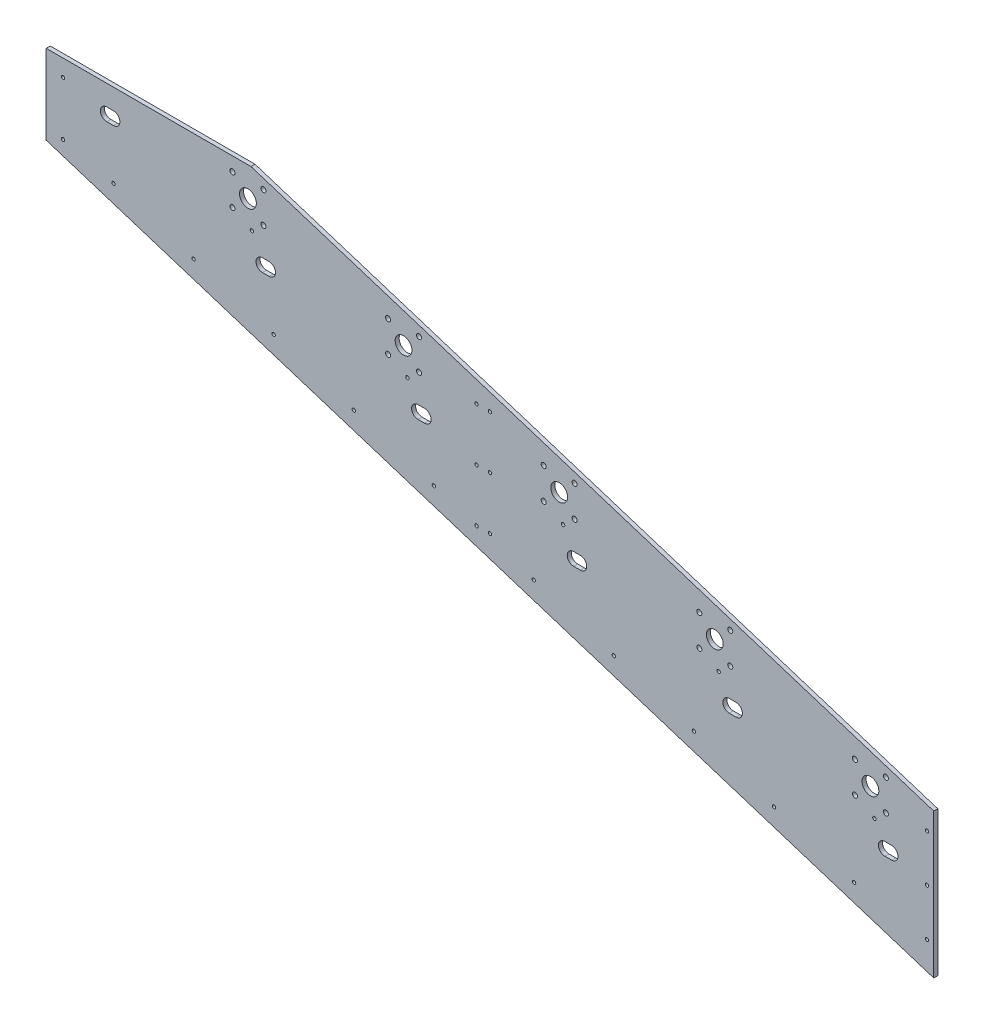
from build123d import *

# Parameters (mm, degrees)
SKETCH_1_W             = 3700
SKETCH_1_H             = 1176
EXTRUDE_1_DEPTH        = 12
SKETCH_2_R             = 19
SKETCH_2_R_2           = 25
CUT_EXTRUDE_1_DEPTH    = 4036.525368524
PATTERN_LINEAR_1_COUNT = 5
PATTERN_LINEAR_1_PITCH = 485.711841895
CUT_EXTRUDE_2_DEPTH    = 4036.525368524
CUT_EXTRUDE_4_DEPTH    = 4036.525368524
CUT_EXTRUDE_5_DEPTH    = 4036.525368524
PATTERN_LINEAR_2_COUNT = 6
PATTERN_LINEAR_2_PITCH = 485.711841895
SKETCH_9_R             = 7.5
CUT_EXTRUDE_11_DEPTH   = 4036.525368524
SKETCH_11_R            = 5
CUT_EXTRUDE_12_DEPTH   = 4036.525368524
PATTERN_LINEAR_3_COUNT = 5
PATTERN_LINEAR_3_PITCH = 485.711841895
SKETCH_12_R            = 5
CUT_EXTRUDE_13_DEPTH   = 3093.743927324
PATTERN_LINEAR_4_COUNT = 5
PATTERN_LINEAR_4_PITCH = 485.711841895
EXTRUDE_4_DEPTH        = 12
CUT_EXTRUDE_14_DEPTH   = 3093.743927324
PATTERN_LINEAR_5_COUNT = 4
PATTERN_LINEAR_5_PITCH = 485.711841895


with BuildPart() as part:
    # 草图1 → 凸台-拉伸1 (new body)
    with BuildSketch(Plane.XY.offset(-510)):
        with Locations((1850, 1023)):
            Rectangle(SKETCH_1_W, SKETCH_1_H)
    extrude(amount=EXTRUDE_1_DEPTH)

    # 草图2 → 切除-拉伸1 (cut, through all)
    with BuildSketch(Plane(origin=(0, 0, -510), x_dir=(-1, 0, 0), z_dir=(0, 0, -1))):
        with Locations((-200, 1531)):
            Circle(SKETCH_2_R)
        with Locations((-599.939078063, 1524.019037425)):
            Circle(SKETCH_2_R_2)
    cut_extrude_1 = extrude(amount=-CUT_EXTRUDE_1_DEPTH, mode=Mode.SUBTRACT)

    # 阵列(线性)1: 切除-拉伸1 ×5
    with Locations(*[Vector(0.9531146620938385, -0.30260938667157716, 0) * (i * PATTERN_LINEAR_1_PITCH) for i in range(1, PATTERN_LINEAR_1_COUNT)]):
        add(cut_extrude_1, mode=Mode.SUBTRACT)

    # 草图5 → 切除-拉伸2 (cut, through all)
    with BuildSketch(Plane(origin=(0, 0, -510), x_dir=(-1, 0, 0), z_dir=(0, 0, -1))):
        Polygon((-608.945764682, 1611), (-3700, 629.604934412), (-3700, 1611), align=None)
    extrude(amount=-CUT_EXTRUDE_2_DEPTH, mode=Mode.SUBTRACT)

    # 草图6 → 切除-拉伸4 (cut, through all)
    with BuildSketch(Plane(origin=(0, 0, -510), x_dir=(-1, 0, 0), z_dir=(0, 0, -1))):
        Polygon((-2958.056115955, 435), (0, 1374.16879321), (0, 435), align=None)
    extrude(amount=-CUT_EXTRUDE_4_DEPTH, mode=Mode.SUBTRACT)

    # 草图7 → 切除-拉伸5 (cut, through all)
    with BuildSketch(Plane(origin=(0, 0, -510), x_dir=(-1, 0, 0), z_dir=(0, 0, -1))):
        with BuildLine():
            Line((-200, 1550), (-180, 1550))
            ThreePointArc((-180, 1550), (-161, 1531), (-180, 1512))
            Line((-180, 1512), (-200, 1512))
            ThreePointArc((-200, 1512), (-219, 1531), (-200, 1550))
        make_face()
    cut_extrude_5 = extrude(amount=-CUT_EXTRUDE_5_DEPTH, mode=Mode.SUBTRACT)

    # 阵列(线性)2: 切除-拉伸5 ×6
    with Locations(*[Vector(0.9531146620938385, -0.30260938667157716, 0) * (i * PATTERN_LINEAR_2_PITCH) for i in range(1, PATTERN_LINEAR_2_COUNT)]):
        add(cut_extrude_5, mode=Mode.SUBTRACT)

    # 草图9 → 切除-拉伸11 (cut, through all)
    with BuildSketch(Plane(origin=(0, 0, -510), x_dir=(-1, 0, 0), z_dir=(0, 0, -1))):
        with Locations((-553.939078063, 1570.019037425)):
            Circle(SKETCH_9_R)
        with Locations((-645.939078063, 1570.019037425)):
            Circle(SKETCH_9_R)
        with Locations((-645.939078063, 1478.019037425)):
            Circle(SKETCH_9_R)
        with Locations((-553.939078063, 1478.019037425)):
            Circle(SKETCH_9_R)
    cut_extrude_11 = extrude(amount=-CUT_EXTRUDE_11_DEPTH, mode=Mode.SUBTRACT)

    # 草图11 → 切除-拉伸12 (cut, through all)
    with BuildSketch(Plane(origin=(0, 0, -510), x_dir=(-1, 0, 0), z_dir=(0, 0, -1))):
        with Locations((-2403.114662094, 663.650866112)):
            Circle(SKETCH_11_R)
        with Locations((-50, 1561)):
            Circle(SKETCH_11_R)
        with Locations((-50, 1401)):
            Circle(SKETCH_11_R)
        with Locations((-200, 1363.129326761)):
            Circle(SKETCH_11_R)
        with Locations((-438.278665523, 1287.476980093)):
            Circle(SKETCH_11_R)
        with Locations((-676.557331047, 1211.824633425)):
            Circle(SKETCH_11_R)
        with Locations((-914.83599657, 1136.172286757)):
            Circle(SKETCH_11_R)
        with Locations((-1153.114662094, 1060.519940089)):
            Circle(SKETCH_11_R)
        with Locations((-1280, 1021)):
            Circle(SKETCH_11_R)
        with Locations((-1320, 1021)):
            Circle(SKETCH_11_R)
        with Locations((-1280, 1178)):
            Circle(SKETCH_11_R)
        with Locations((-1320, 1178)):
            Circle(SKETCH_11_R)
        with Locations((-1320, 1335)):
            Circle(SKETCH_11_R)
        with Locations((-1280, 1335)):
            Circle(SKETCH_11_R)
        with Locations((-1450, 966.260252783)):
            Circle(SKETCH_11_R)
        with Locations((-1688.278665523, 890.607906115)):
            Circle(SKETCH_11_R)
        with Locations((-1926.557331047, 814.955559447)):
            Circle(SKETCH_11_R)
        with Locations((-2164.83599657, 739.30321278)):
            Circle(SKETCH_11_R)
        with Locations((-2620, 625)):
            Circle(SKETCH_11_R)
        with Locations((-2620, 765)):
            Circle(SKETCH_11_R)
        with Locations((-2620, 905)):
            Circle(SKETCH_11_R)
    extrude(amount=-CUT_EXTRUDE_12_DEPTH, mode=Mode.SUBTRACT)

    # 阵列(线性)3: 切除-拉伸11 ×5
    with Locations(*[Vector(0.9531146620938385, -0.30260938667157716, 0) * (i * PATTERN_LINEAR_3_PITCH) for i in range(1, PATTERN_LINEAR_3_COUNT)]):
        add(cut_extrude_11, mode=Mode.SUBTRACT)

    # Surface Cut 1
    split(bisect_by=Plane.ZY.offset(-2640), keep=Keep.TOP)

    # 草图12 → 切除-拉伸13 (cut, through all)
    with BuildSketch(Plane(origin=(0, 0, -510), x_dir=(-1, 0, 0), z_dir=(0, 0, -1))):
        with Locations((-611.679078063, 1446.789037425)):
            Circle(SKETCH_12_R)
    cut_extrude_13 = extrude(amount=-CUT_EXTRUDE_13_DEPTH, mode=Mode.SUBTRACT)

    # 阵列(线性)4: 切除-拉伸13 ×5
    with Locations(*[Vector(0.9531146620938385, -0.3026093866715771, 0) * (i * PATTERN_LINEAR_4_PITCH) for i in range(1, PATTERN_LINEAR_4_COUNT)]):
        add(cut_extrude_13, mode=Mode.SUBTRACT)

    # 草图15 → 凸台-拉伸4 (add, through all)
    with BuildSketch(Plane(origin=(0, 0, -510), x_dir=(-1, 0, 0), z_dir=(0, 0, -1))):
        with BuildLine():
            Line((-662.939078063, 1414.019037425), (-642.939078063, 1414.019037425))
            ThreePointArc((-642.939078063, 1414.019037425), (-612.939078063, 1384.019037425), (-642.939078063, 1354.019037425))
            Line((-642.939078063, 1354.019037425), (-662.939078063, 1354.019037425))
            ThreePointArc((-662.939078063, 1354.019037425), (-692.939078063, 1384.019037425), (-662.939078063, 1414.019037425))
        make_face()
        with BuildLine():
            Line((-1125.878156125, 1267.03807485), (-1105.878156125, 1267.03807485))
            ThreePointArc((-1105.878156125, 1267.03807485), (-1075.878156125, 1237.03807485), (-1105.878156125, 1207.03807485))
            Line((-1105.878156125, 1207.03807485), (-1125.878156125, 1207.03807485))
            ThreePointArc((-1125.878156125, 1207.03807485), (-1155.878156125, 1237.03807485), (-1125.878156125, 1267.03807485))
        make_face()
        with BuildLine():
            Line((-1588.817234188, 1120.057112275), (-1568.817234188, 1120.057112275))
            ThreePointArc((-1568.817234188, 1120.057112275), (-1538.817234188, 1090.057112275), (-1568.817234188, 1060.057112275))
            Line((-1568.817234188, 1060.057112275), (-1588.817234188, 1060.057112275))
            ThreePointArc((-1588.817234188, 1060.057112275), (-1618.817234188, 1090.057112275), (-1588.817234188, 1120.057112275))
        make_face()
        with BuildLine():
            Line((-2051.75631225, 973.0761497), (-2031.75631225, 973.0761497))
            ThreePointArc((-2031.75631225, 973.0761497), (-2001.75631225, 943.0761497), (-2031.75631225, 913.0761497))
            Line((-2031.75631225, 913.0761497), (-2051.75631225, 913.0761497))
            ThreePointArc((-2051.75631225, 913.0761497), (-2081.75631225, 943.0761497), (-2051.75631225, 973.0761497))
        make_face()
    extrude(amount=-EXTRUDE_4_DEPTH)

    # 草图14 → 切除-拉伸14 (cut, through all)
    with BuildSketch(Plane(origin=(0, 0, -510), x_dir=(-1, 0, 0), z_dir=(0, 0, -1))):
        with BuildLine():
            Line((-642.939078063, 1393.019037425), (-662.939078063, 1393.019037425))
            ThreePointArc((-662.939078063, 1393.019037425), (-681.939078063, 1374.019037425), (-662.939078063, 1355.019037425))
            Line((-662.939078063, 1355.019037425), (-642.939078063, 1355.019037425))
            ThreePointArc((-642.939078063, 1355.019037425), (-623.939078063, 1374.019037425), (-642.939078063, 1393.019037425))
        make_face()
    cut_extrude_14 = extrude(amount=-CUT_EXTRUDE_14_DEPTH, mode=Mode.SUBTRACT)

    # 阵列(线性)5: 切除-拉伸14 ×4
    with Locations(*[Vector(0.9531146620938385, -0.3026093866715771, 0) * (i * PATTERN_LINEAR_5_PITCH) for i in range(1, PATTERN_LINEAR_5_COUNT)]):
        add(cut_extrude_14, mode=Mode.SUBTRACT)


solid = part.part
